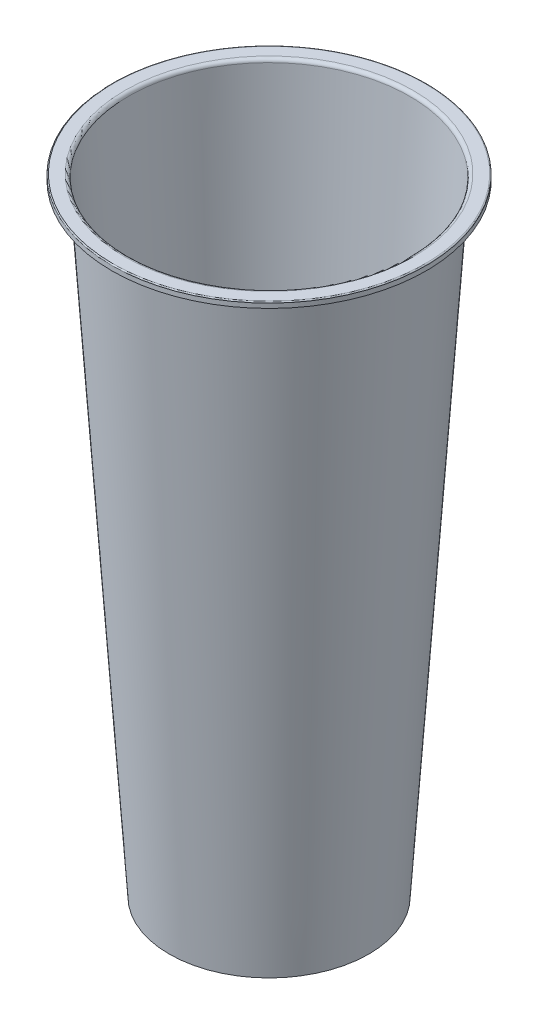
from build123d import *


with BuildPart() as part:
    # 草图1 → 旋转1 (revolve)
    with BuildSketch(Plane.XY, mode=Mode.PRIVATE) as revolve_1_sk:
        with BuildLine():
            Line((-44.2, 177), (-40.83502586, 177))
            ThreePointArc((-40.83502586, 177), (-40.152047165, 176.730438295), (-39.837278274, 176.067080205))
            Line((-39.837278274, 176.067080205), (-28, 0))
            Line((-28, 0), (0, 0))
            Line((0, 0), (0, -0.3))
            Line((0, -0.3), (-28.280507758, -0.3))
            Line((-28.280507758, -0.3), (-40.13660255, 176.046956143))
            ThreePointArc((-40.13660255, 176.046956143), (-40.356940774, 176.511306806), (-40.83502586, 176.7))
            Line((-40.83502586, 176.7), (-44.2, 176.7))
            Line((-44.2, 176.7), (-44.2, 175.4))
            Line((-44.2, 175.4), (-44.5, 175.4))
            Line((-44.5, 175.4), (-44.5, 176.7))
            ThreePointArc((-44.5, 176.7), (-44.412132034, 176.912132034), (-44.2, 177))
        make_face()
    revolve(revolve_1_sk.sketch.rotate(Axis((0, 0, 0), (0, -1, 0)), 270), axis=Axis((0, 0, 0), (0, -1, 0)))


solid = part.part
